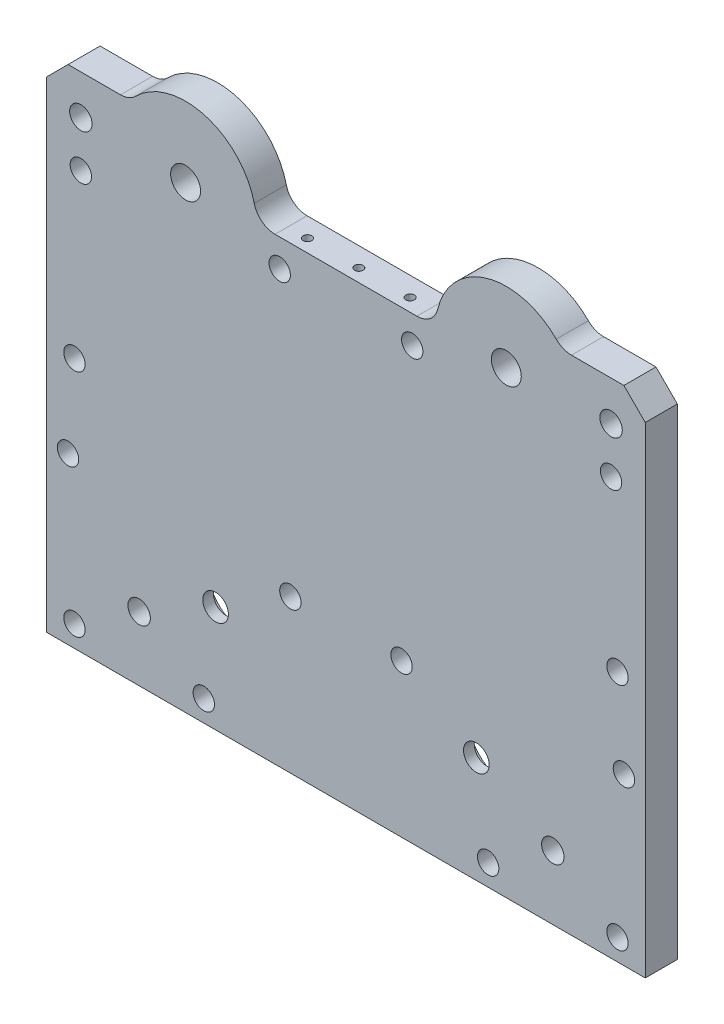
from build123d import *

# Parameters (mm, degrees)
BOSS_EXTRUDE1_DEPTH     = 5
SKETCH10_W              = 430.19860944
SKETCH10_H              = 431.937312902
SKETCH10_W_2            = 300
SKETCH10_H_2            = 230
CUT_EXTRUDE1_DEPTH      = 50
CUT_EXTRUDE2_DEPTH      = 34
CUT_EXTRUDE2_DEPTH_BACK = 67
SKETCH11_R              = 7
CUT_EXTRUDE3_DEPTH      = 83
CUT_EXTRUDE3_DEPTH_BACK = 62
SKETCH13_W              = 90
SKETCH13_H              = 26.63854706
CUT_EXTRUDE4_DEPTH      = 38
SKETCH16_R              = 6
CUT_EXTRUDE7_DEPTH      = 36
CUT_EXTRUDE8_DEPTH      = 10
BOSS_EXTRUDE2_DEPTH     = 10
SKETCH23_W              = 266
SKETCH23_H              = 30
BOSS_EXTRUDE5_DEPTH     = 15
SKETCH24_W              = 32
SKETCH24_H              = 53.383916467
CUT_EXTRUDE9_DEPTH      = 10
BOSS_EXTRUDE6_DEPTH     = 10
CUT_EXTRUDE10_DEPTH     = 56
CUT_EXTRUDE11_DEPTH     = 15
CUT_EXTRUDE12_DEPTH     = 10
BOSS_EXTRUDE7_START     = 10
SKETCH33_R              = 6
SKETCH33_R_2            = 7
BOSS_EXTRUDE7_DEPTH     = 10
CUT_EXTRUDE13_START     = -10
SKETCH32_R              = 6
CUT_EXTRUDE13_DEPTH     = 10
SKETCH34_R              = 3
CUT_EXTRUDE14_DEPTH     = 30
SKETCH36_R              = 3.25
CUT_EXTRUDE15_DEPTH     = 30
SKETCH37_R              = 5
CUT_EXTRUDE18_DEPTH     = 10
BOSS_EXTRUDE8_DEPTH     = 15
CHAMFER1_SIZE           = 10
SKETCH39_R              = 3.25
CUT_EXTRUDE19_DEPTH     = 143
CUT_EXTRUDE20_START     = -10
SKETCH40_R              = 5
SKETCH40_R_2            = 3.25
CUT_EXTRUDE20_DEPTH     = 10
SKETCH41_R              = 7
BOSS_EXTRUDE9_DEPTH     = 15
SKETCH42_R              = 5.25
CUT_EXTRUDE21_DEPTH     = 78
FILLET1_R               = 10
FILLET2_R               = 10
SKETCH43_R              = 3.25
CUT_EXTRUDE22_DEPTH     = 69
SKETCH44_R              = 5
CUT_EXTRUDE23_DEPTH     = 10
SKETCH45_R              = 5
CUT_EXTRUDE24_DEPTH     = 81
SKETCH46_R              = 2
CUT_EXTRUDE26_DEPTH     = 10
SKETCH47_R              = 18.5
SKETCH47_R_2            = 16.5
CUT_EXTRUDE27_DEPTH     = 1.8


with BuildPart() as part:
    # Sketch1 → Boss-Extrude1 (new body)
    with BuildSketch(Plane.XY):
        Polygon((-150, -150), (-150, -170), (150, -170), (150, -150), (150, 150), (-150, 150), align=None)
    extrude(amount=BOSS_EXTRUDE1_DEPTH)

    # Sketch10 → Cut-Extrude1 (cut)
    with BuildSketch(Plane.XY.offset(5)):
        Rectangle(SKETCH10_W, SKETCH10_H)
        with Locations((0, -55)):
            Rectangle(SKETCH10_W_2, SKETCH10_H_2, mode=Mode.SUBTRACT)
    extrude(amount=-CUT_EXTRUDE1_DEPTH, mode=Mode.SUBTRACT)

    # Sketch11 → Cut-Extrude2 (cut, two sides: drawn at the far end of the back side and taken through both)
    with BuildSketch(Plane.XY.offset(5).offset(-CUT_EXTRUDE2_DEPTH_BACK)):
        with Locations(Location((-75, 39.647459622, 0), (0, 0, 180))):
            Circle(SKETCH11_R)
        with Locations(Location((75, 39.647459622, 0), (0, 0, 180))):
            Circle(SKETCH11_R)
    extrude(amount=CUT_EXTRUDE2_DEPTH + CUT_EXTRUDE2_DEPTH_BACK, mode=Mode.SUBTRACT)

    # Sketch12 → Cut-Extrude3 (cut, two sides: drawn at the far end of the back side and taken through both)
    with BuildSketch(Plane.XY.offset(5).offset(-CUT_EXTRUDE3_DEPTH_BACK)):
        Polygon((-150, 60), (-133, 60), (-133, -183.341935532), (-188.985171206, -183.341935532), (-185.209913478, 60), align=None)
        Polygon((185.209913478, 60), (150, 60), (133, 60), (133, -183.341935532), (188.985171206, -183.341935532), align=None)
    extrude(amount=CUT_EXTRUDE3_DEPTH + CUT_EXTRUDE3_DEPTH_BACK, mode=Mode.SUBTRACT)

    # Sketch13 → Cut-Extrude4 (cut)
    with BuildSketch(Plane.XY.offset(5)):
        with Locations((0, 52.966733152)):
            Rectangle(SKETCH13_W, SKETCH13_H)
    extrude(amount=-CUT_EXTRUDE4_DEPTH, mode=Mode.SUBTRACT)

    # Sketch16 → Cut-Extrude7 (cut)
    with BuildSketch(Plane.XY.offset(5)):
        with Locations((-60.989142528, -125.260874967)):
            Circle(SKETCH16_R)
        with Locations((60.989142528, -125.260874967)):
            Circle(SKETCH16_R)
    extrude(amount=-CUT_EXTRUDE7_DEPTH, mode=Mode.SUBTRACT)

    # Sketch18 → Cut-Extrude8 (cut)
    with BuildSketch(Plane.XY.offset(5)):
        Polygon((-63.637907567, -145.025157671), (138.825867156, -145.025157671), (138.825867156, -178.761284058), (-147.679626059, -178.761284058), (-147.679626059, -145.025157671), align=None)
    extrude(amount=-CUT_EXTRUDE8_DEPTH, mode=Mode.SUBTRACT)

    # Sketch20 → Boss-Extrude2 (add)
    with BuildSketch(Plane.XY.offset(5)):
        Polygon((-119.231997115, -76.857332264), (-119.231997115, -50.797544119), (-130, -50.797544119), (-130, -19.723575517), (-108, -19.723575517), (-108, 60), (-133, 20), (-133, -145.025157671), (133, -145.025157671), (133, 20), (108, 60), (108, -19.723575517), (130, -19.723575517), (130, -50.797544119), (119.231997115, -50.797544119), (119.231997115, -76.857332264), (119.231997115, -125.260874967), (80.989142528, -125.260874967), (80.989142528, -142.025157671), (40.835190362, -142.025157671), (40.835190362, -125.260874967), (-40.835190362, -125.260874967), (-40.835190362, -142.025157671), (-80.989142528, -142.025157671), (-80.989142528, -125.260874967), (-119.231997115, -125.260874967), align=None)
    extrude(amount=BOSS_EXTRUDE2_DEPTH)

    # Sketch23 → Boss-Extrude5 (add)
    with BuildSketch(Plane.XY.offset(15)):
        with Locations((0, -160.025157671)):
            Rectangle(SKETCH23_W, SKETCH23_H)
    extrude(amount=-BOSS_EXTRUDE5_DEPTH)

    # Sketch24 → Cut-Extrude9 (cut)
    with BuildSketch(Plane.XY.offset(15)):
        with Locations((0, -151.952833201)):
            Rectangle(SKETCH24_W, SKETCH24_H)
    extrude(amount=-CUT_EXTRUDE9_DEPTH, mode=Mode.SUBTRACT)

    # Sketch25 → Boss-Extrude6 (add)
    with BuildSketch(Plane.XY.offset(15)):
        with BuildLine():
            Line((-77.989142528, -125.260874967), (-80.989142528, -125.260874967))
            Line((-80.989142528, -125.260874967), (-80.989142528, -142.025157671))
            Line((-80.989142528, -142.025157671), (-63.810281555, -142.025157671))
            ThreePointArc((-63.810281555, -142.025157671), (-73.969114859, -136.239049599), (-77.989142528, -125.260874967))
        make_face()
        with BuildLine():
            Line((-58.1680035, -142.025157671), (-40.835190362, -142.025157671))
            Line((-40.835190362, -142.025157671), (-40.835190362, -125.260874967))
            Line((-40.835190362, -125.260874967), (-43.989142528, -125.260874967))
            ThreePointArc((-43.989142528, -125.260874967), (-48.009170196, -136.239049599), (-58.1680035, -142.025157671))
        make_face()
        with BuildLine():
            Line((40.835190362, -125.260874967), (43.989142528, -125.260874967))
            ThreePointArc((43.989142528, -125.260874967), (48.009170196, -136.239049599), (58.1680035, -142.025157671))
            Line((58.1680035, -142.025157671), (40.835190362, -142.025157671))
            Line((40.835190362, -142.025157671), (40.835190362, -125.260874967))
        make_face()
        with BuildLine():
            Line((80.989142528, -142.025157671), (63.810281555, -142.025157671))
            ThreePointArc((63.810281555, -142.025157671), (73.969114859, -136.239049599), (77.989142528, -125.260874967))
            Line((77.989142528, -125.260874967), (80.989142528, -125.260874967))
            Line((80.989142528, -125.260874967), (80.989142528, -142.025157671))
        make_face()
    extrude(amount=-BOSS_EXTRUDE6_DEPTH)

    # Sketch28 → Cut-Extrude10 (cut)
    with BuildSketch(Plane.XY.offset(5)):
        Polygon((-46, 60), (-41.318426322, 60), (-41.318426322, 39.647459622), (-46, 39.647459622), (-66, 60), align=None)
        Polygon((41.318426322, 39.647459622), (46, 39.647459622), (66, 60), (46, 60), (41.318426322, 60), align=None)
    extrude(amount=-CUT_EXTRUDE10_DEPTH, mode=Mode.SUBTRACT)

    # Sketch29 → Cut-Extrude11 (cut)
    with BuildSketch(Plane.XY.offset(5)):
        Polygon((-133, 60), (-133, 20), (-108, 60), align=None)
        Polygon((108, 60), (133, 20), (133, 60), align=None)
    extrude(amount=-CUT_EXTRUDE11_DEPTH, mode=Mode.SUBTRACT)

    # Sketch31 → Cut-Extrude12 (cut)
    with BuildSketch(Plane.XY.offset(15)):
        Polygon((-108, 35), (-130, -19.723575517), (-94.809291049, -33.870962445), align=None)
        Polygon((108, 35), (130, -19.723575517), (80.731863312, -35.260559818), align=None)
    extrude(amount=-CUT_EXTRUDE12_DEPTH, mode=Mode.SUBTRACT)

    # Sketch33 → Boss-Extrude7 (add)
    with BuildSketch(Plane.XY.offset(5).offset(BOSS_EXTRUDE7_START)):
        Polygon((-66, 60), (-46, 39.647459622), (46, 39.647459622), (66, 60), (108, 60), (133, 20), (133, -175.025157671), (16, -175.025157671), (-16, -175.025157671), (-133, -175.025157671), (-133, 20), (-108, 60), align=None)
        with Locations((60.989142528, -125.260874967)):
            Circle(SKETCH33_R, mode=Mode.SUBTRACT)
        with Locations((-60.989142528, -125.260874967)):
            Circle(SKETCH33_R, mode=Mode.SUBTRACT)
        with Locations(Location((75, 39.647459622, 0), (0, 0, 180))):
            Circle(SKETCH33_R_2, mode=Mode.SUBTRACT)
        with Locations(Location((-75, 39.647459622, 0), (0, 0, 180))):
            Circle(SKETCH33_R_2, mode=Mode.SUBTRACT)
    extrude(amount=-BOSS_EXTRUDE7_DEPTH)

    # Sketch32 → Cut-Extrude13 (cut)
    # profile 1 of 2: a face of its own
    with BuildSketch(Plane(origin=(0, 0, 0), x_dir=(-1, 0, 0), z_dir=(0, 0, -1)).offset(CUT_EXTRUDE13_START)):
        with BuildLine():
            Line((-67.822136157, 20.740397673), (-95.527284672, 16.361527024))
            ThreePointArc((-95.527284672, 16.361527024), (-109.101071589, 6.94486247), (-110.170402891, -9.540822021))
            Line((-110.170402891, -9.540822021), (-80.481739168, -82.809756918))
            Line((-80.481739168, -82.809756918), (-79.981902791, -124.736415651))
            ThreePointArc((-79.981902791, -124.736415651), (-62.46056345, -144.203813505), (-42.143210868, -127.67559232))
            Line((-42.143210868, -127.67559232), (-35.693180555, -83.14547495))
            Line((-35.693180555, -83.14547495), (-14.837962686, -27.195571485))
            ThreePointArc((-14.837962686, -27.195571485), (-14.285820116, -14.579696177), (-21.763980146, -4.404122789))
            Line((-21.763980146, -4.404122789), (-54.154979556, 17.673328836))
            ThreePointArc((-54.154979556, 17.673328836), (-60.695607968, 20.512276405), (-67.822136157, 20.740397673))
        make_face()
        with Locations(Location((-60.989142528, -125.260874967, 0), (0, 0, 180))):
            Circle(SKETCH32_R, mode=Mode.SUBTRACT)
    # profile 2 of 2: a face of its own
    with BuildSketch(Plane(origin=(0, 0, 0), x_dir=(-1, 0, 0), z_dir=(0, 0, -1)).offset(CUT_EXTRUDE13_START)):
        with BuildLine():
            Line((54.154979556, 17.673328836), (21.763980146, -4.404122789))
            ThreePointArc((21.763980146, -4.404122789), (14.285820116, -14.579696177), (14.837962686, -27.195571485))
            Line((14.837962686, -27.195571485), (35.693180555, -83.14547495))
            Line((35.693180555, -83.14547495), (42.143210868, -127.67559232))
            ThreePointArc((42.143210868, -127.67559232), (62.46056345, -144.203813505), (79.981902791, -124.736415651))
            Line((79.981902791, -124.736415651), (80.481739168, -82.809756918))
            Line((80.481739168, -82.809756918), (110.170402891, -9.540822021))
            ThreePointArc((110.170402891, -9.540822021), (109.101071589, 6.94486247), (95.527284672, 16.361527024))
            Line((95.527284672, 16.361527024), (67.822136157, 20.740397673))
            ThreePointArc((67.822136157, 20.740397673), (60.695607968, 20.512276405), (54.154979556, 17.673328836))
        make_face()
        with Locations(Location((60.989142528, -125.260874967, 0), (0, 0, 180))):
            Circle(SKETCH32_R, mode=Mode.SUBTRACT)
    extrude(amount=CUT_EXTRUDE13_DEPTH, mode=Mode.SUBTRACT)

    # Sketch34 → Cut-Extrude14 (cut)
    with BuildSketch(Plane.XZ.offset(175.025157671)):
        with Locations(Location((23.5, 8.5, 0), (0, 0, 270))):
            Circle(SKETCH34_R)
        with Locations(Location((-23.5, 8.5, 0), (0, 0, 270))):
            Circle(SKETCH34_R)
    extrude(amount=-CUT_EXTRUDE14_DEPTH, mode=Mode.SUBTRACT)

    # Sketch36 → Cut-Extrude15 (cut)
    with BuildSketch(Plane.XY.offset(15)):
        with Locations((-124, 20)):
            Circle(SKETCH36_R)
        with Locations((-127, -57.512578835)):
            Circle(SKETCH36_R)
        with Locations((-127, -165.025157671)):
            Circle(SKETCH36_R)
        with Locations((-66.5, -165.025157671)):
            Circle(SKETCH36_R)
        with Locations((66.5, -165.025157671)):
            Circle(SKETCH36_R)
        with Locations((127, -165.025157671)):
            Circle(SKETCH36_R)
        with Locations((127, -57.512578835)):
            Circle(SKETCH36_R)
        with Locations((124, 20)):
            Circle(SKETCH36_R)
    extrude(amount=-CUT_EXTRUDE15_DEPTH, mode=Mode.SUBTRACT)

    # Sketch37 → Cut-Extrude18 (cut)
    with BuildSketch(Plane.XY.offset(15)):
        with Locations((-124, 20)):
            Circle(SKETCH37_R)
        with Locations((-127, -57.512578835)):
            Circle(SKETCH37_R)
        with Locations((-127, -165.025157671)):
            Circle(SKETCH37_R)
        with Locations((-66.5, -165.025157671)):
            Circle(SKETCH37_R)
        with Locations((66.5, -165.025157671)):
            Circle(SKETCH37_R)
        with Locations((127, -165.025157671)):
            Circle(SKETCH37_R)
        with Locations((127, -57.512578835)):
            Circle(SKETCH37_R)
        with Locations((124, 20)):
            Circle(SKETCH37_R)
    extrude(amount=-CUT_EXTRUDE18_DEPTH, mode=Mode.SUBTRACT)

    # Sketch38 → Boss-Extrude8 (add)
    with BuildSketch(Plane.XY.offset(15)):
        Polygon((108, 60), (140, 60), (140, -175.025157671), (133, -175.025157671), (133, 20), align=None)
        Polygon((-108, 60), (-133, 20), (-133, -175.025157671), (-140, -175.025157671), (-140, 60), align=None)
    extrude(amount=-BOSS_EXTRUDE8_DEPTH)

    # Chamfer1
    chamfer1_edges = [part.edges().sort_by_distance(p)[0] for p in [
        (140, 60, 7.5),
        (-140, 60, 7.5),
    ]]
    chamfer(chamfer1_edges, length=CHAMFER1_SIZE)

    # Sketch39 → Cut-Extrude19 (cut)
    with BuildSketch(Plane(origin=(0, 0, 0), x_dir=(-1, 0, 0), z_dir=(0, 0, -1))):
        with Locations((-31, 26.672459622)):
            Circle(SKETCH39_R)
        with Locations((31, 26.672459622)):
            Circle(SKETCH39_R)
    extrude(amount=-CUT_EXTRUDE19_DEPTH, mode=Mode.SUBTRACT)

    # Sketch40 → Cut-Extrude20 (cut)
    # profile 1 of 2: a face of its own
    with BuildSketch(Plane.XY.offset(15).offset(CUT_EXTRUDE20_START)):
        with Locations((31, 26.672459622)):
            Circle(SKETCH40_R)
        with Locations(Location((31, 26.672459622, 0), (0, 0, 180))):
            Circle(SKETCH40_R_2, mode=Mode.SUBTRACT)
    # profile 2 of 2: a face of its own
    with BuildSketch(Plane.XY.offset(15).offset(CUT_EXTRUDE20_START)):
        with Locations((-31, 26.672459622)):
            Circle(SKETCH40_R)
    extrude(amount=CUT_EXTRUDE20_DEPTH, mode=Mode.SUBTRACT)

    # Sketch41 → Boss-Extrude9 (add)
    # profile 1 of 2: a face of its own
    with BuildSketch(Plane.XY.offset(15)):
        with BuildLine():
            Line((106.336958161, 29.303618305), (43.663041839, 29.303618305))
            ThreePointArc((43.663041839, 29.303618305), (75, 72.647459622), (106.336958161, 29.303618305))
        make_face()
        with Locations(Location((75, 39.647459622, 0), (0, 0, 180))):
            Circle(SKETCH41_R, mode=Mode.SUBTRACT)
    # profile 2 of 2: a face of its own
    with BuildSketch(Plane.XY.offset(15)):
        with BuildLine():
            Line((-106.336958161, 29.303618305), (-43.663041839, 29.303618305))
            ThreePointArc((-43.663041839, 29.303618305), (-75, 72.647459622), (-106.336958161, 29.303618305))
        make_face()
        with Locations(Location((-75, 39.647459622, 0), (0, 0, 180))):
            Circle(SKETCH41_R, mode=Mode.SUBTRACT)
    extrude(amount=-BOSS_EXTRUDE9_DEPTH)

    # Sketch42 → Cut-Extrude21 (cut)
    with BuildSketch(Plane(origin=(0, 0, 0), x_dir=(-1, 0, 0), z_dir=(0, 0, -1))):
        with Locations((124, 41.5)):
            Circle(SKETCH42_R)
        with Locations((-124, 41.5)):
            Circle(SKETCH42_R)
        with Locations((-96.75, -145.025157671)):
            Circle(SKETCH42_R)
        with Locations((96.75, -145.025157671)):
            Circle(SKETCH42_R)
    extrude(amount=-CUT_EXTRUDE21_DEPTH, mode=Mode.SUBTRACT)

    # Fillet1
    fillet1_edges = [part.edges().sort_by_distance(p)[0] for p in [
        (42, 39.647459622, 7.5),
        (-42, 39.647459622, 7.5),
    ]]
    fillet(fillet1_edges, radius=FILLET1_R)

    # Fillet2
    fillet2_edges = [part.edges().sort_by_distance(p)[0] for p in [
        (100.976414305, 60, 7.5),
        (-100.976414305, 60, 7.5),
    ]]
    fillet(fillet2_edges, radius=FILLET2_R)

    # Sketch43 → Cut-Extrude22 (cut)
    with BuildSketch(Plane.XY.offset(15)):
        with Locations((26, -103.513035633)):
            Circle(SKETCH43_R)
        with Locations((-26, -103.513035633)):
            Circle(SKETCH43_R)
    extrude(amount=-CUT_EXTRUDE22_DEPTH, mode=Mode.SUBTRACT)

    # Sketch44 → Cut-Extrude23 (cut)
    with BuildSketch(Plane.XY.offset(15)):
        with Locations((-26, -103.513035633)):
            Circle(SKETCH44_R)
        with Locations((26, -103.513035633)):
            Circle(SKETCH44_R)
    extrude(amount=-CUT_EXTRUDE23_DEPTH, mode=Mode.SUBTRACT)

    # Sketch45 → Cut-Extrude24 (cut)
    with BuildSketch(Plane(origin=(0, 0, 0), x_dir=(-1, 0, 0), z_dir=(0, 0, -1))):
        with Locations((130.000000029, -97.512578887)):
            Circle(SKETCH45_R)
        with Locations((-129.999999971, -97.512578887)):
            Circle(SKETCH45_R)
    extrude(amount=-CUT_EXTRUDE24_DEPTH, mode=Mode.SUBTRACT)

    # Sketch46 → Cut-Extrude26 (cut)
    with BuildSketch(Plane(origin=(0, 39.647459622, 0), x_dir=(1, 0, 0), z_dir=(0, 1, 0))):
        with Locations(Location((-24, -9, 0), (0, 0, 180))):
            Circle(SKETCH46_R)
        with Locations(Location((0, -9, 0), (0, 0, 180))):
            Circle(SKETCH46_R)
        with Locations(Location((24, -9, 0), (0, 0, 180))):
            Circle(SKETCH46_R)
    extrude(amount=-CUT_EXTRUDE26_DEPTH, mode=Mode.SUBTRACT)

    # Sketch47 → Cut-Extrude27 (cut)
    # profile 1 of 2: a face of its own
    with BuildSketch(Plane(origin=(0, 0, 0), x_dir=(-1, 0, 0), z_dir=(0, 0, -1))):
        with Locations((-75, 39.647459622)):
            Circle(SKETCH47_R)
        with Locations((-75, 39.647459622)):
            Circle(SKETCH47_R_2, mode=Mode.SUBTRACT)
    # profile 2 of 2: a face of its own
    with BuildSketch(Plane(origin=(0, 0, 0), x_dir=(-1, 0, 0), z_dir=(0, 0, -1))):
        with Locations((75, 39.647459622)):
            Circle(SKETCH47_R)
        with Locations((75, 39.647459622)):
            Circle(SKETCH47_R_2, mode=Mode.SUBTRACT)
    extrude(amount=-CUT_EXTRUDE27_DEPTH, mode=Mode.SUBTRACT)


solid = part.part
